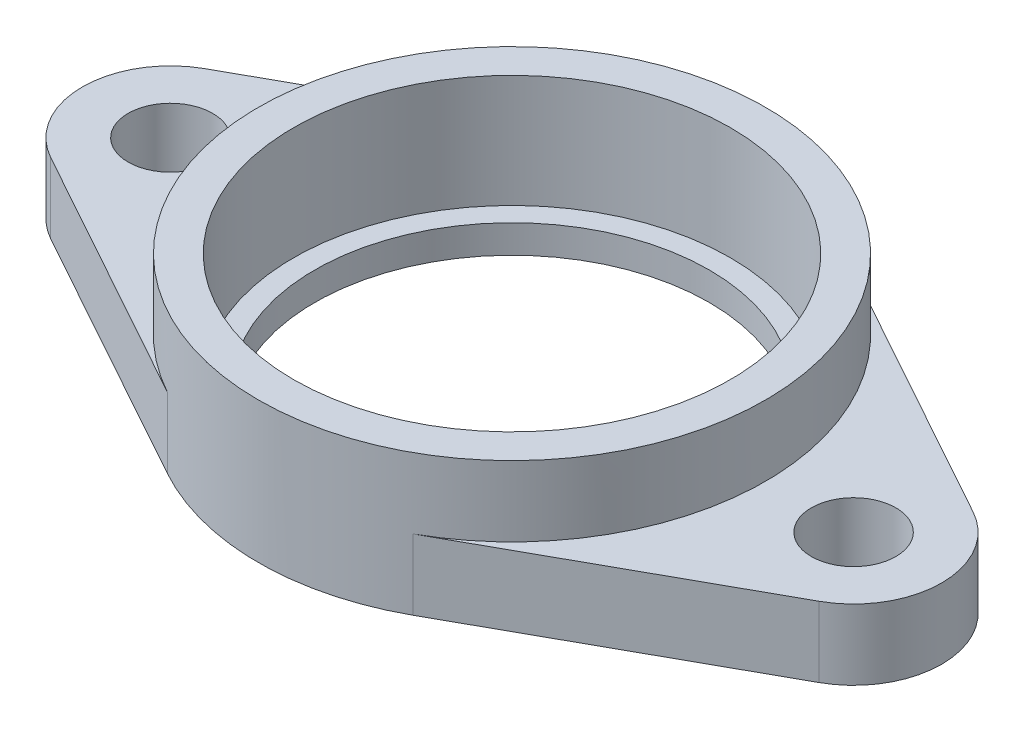
from build123d import *

# Parameters (mm, degrees)
SKETCH_1_R          = 6
EXTRUDE_1_DEPTH     = 10
SKETCH_2_R          = 36
EXTRUDE_2_DEPTH     = 10
SKETCH_3_R          = 31
CUT_EXTRUDE_1_DEPTH = 16
SKETCH_4_R          = 28
CUT_EXTRUDE_2_DEPTH = 16


with BuildPart() as part:
    # 草图1 → 凸台-拉伸1 (new body)
    with BuildSketch(Plane(origin=(0, 0, 0), x_dir=(1, 0, 0), z_dir=(0, 1, 0))):
        with BuildLine():
            Line((-54.556701031, 10.934640946), (-17.443298969, 31.491765925))
            ThreePointArc((-17.443298969, 31.491765925), (0, 36), (17.443298969, 31.491765925))
            Line((17.443298969, 31.491765925), (54.556701031, 10.934640946))
            ThreePointArc((54.556701031, 10.934640946), (61, 0), (54.556701031, -10.934640946))
            Line((54.556701031, -10.934640946), (17.443298969, -31.491765925))
            ThreePointArc((17.443298969, -31.491765925), (0, -36), (-17.443298969, -31.491765925))
            Line((-17.443298969, -31.491765925), (-54.556701031, -10.934640946))
            ThreePointArc((-54.556701031, -10.934640946), (-61, 0), (-54.556701031, 10.934640946))
        make_face()
        with Locations(Location((48.5, 0, 0), (0, 0, 270))):
            Circle(SKETCH_1_R, mode=Mode.SUBTRACT)
        with Locations(Location((-48.5, 0, 0), (0, 0, 270))):
            Circle(SKETCH_1_R, mode=Mode.SUBTRACT)
    extrude(amount=EXTRUDE_1_DEPTH)

    # 草图2 → 凸台-拉伸2 (add)
    with BuildSketch(Plane(origin=(0, 10, 0), x_dir=(1, 0, 0), z_dir=(0, 1, 0))):
        with Locations(Location((0, 0, 0), (0, 0, 118.982082268))):
            Circle(SKETCH_2_R)
    extrude(amount=EXTRUDE_2_DEPTH)

    # 草图3 → 切除-拉伸1 (cut)
    with BuildSketch(Plane(origin=(0, 20, 0), x_dir=(1, 0, 0), z_dir=(0, 1, 0))):
        with Locations(Location((0, 0, 0), (0, 0, 270))):
            Circle(SKETCH_3_R)
    extrude(amount=-CUT_EXTRUDE_1_DEPTH, mode=Mode.SUBTRACT)

    # 草图4 → 切除-拉伸2 (cut)
    with BuildSketch(Plane(origin=(0, 4, 0), x_dir=(1, 0, 0), z_dir=(0, 1, 0))):
        with Locations(Location((0, 0, 0), (0, 0, 270))):
            Circle(SKETCH_4_R)
    extrude(amount=-CUT_EXTRUDE_2_DEPTH, mode=Mode.SUBTRACT)


solid = part.part
